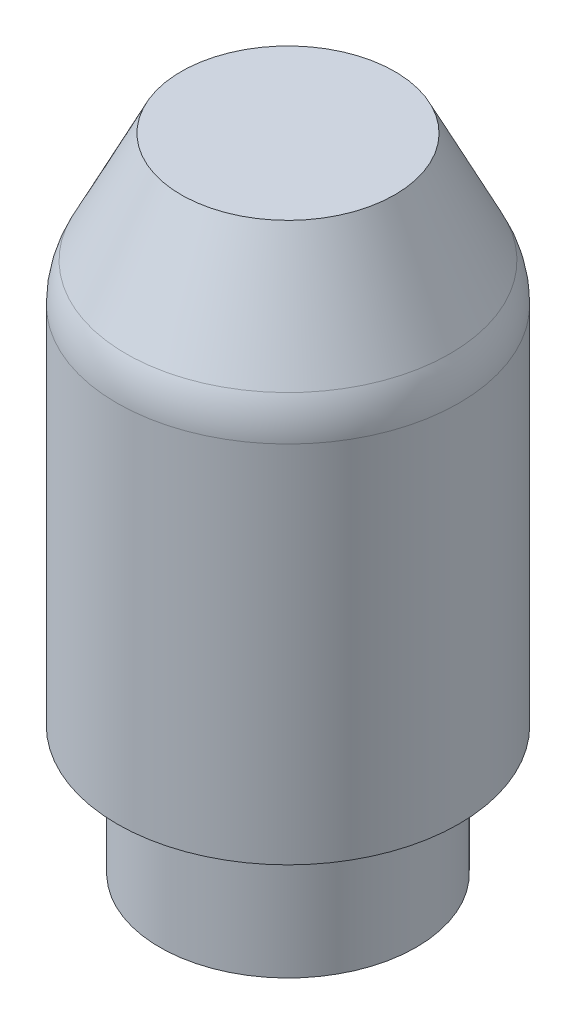
SolidWorks part; units mm, degrees
material "SKD11"
ref_plane "Front Plane" through (0, 0, 0) normal (0, 0, 1) x (1, 0, 0)
ref_plane "Top Plane" through (0, 0, 0) normal (0, 1, 0) x (1, 0, 0)
ref_plane "Right Plane" through (0, 0, 0) normal (1, 0, 0) x (0, 0, -1)
sketch "Sketch1" plane through (0, 0, 0) normal (0, 0, 1) x (1, 0, 0)
  line L0 (0, 0) -> (0, 15)
  line L1 (0, 15) -> (2.5, 15)
  line L2 (4, 12) -> (4, 3)
  line L3 (3, 0) -> (0, 0)
  line L4 (2.5, 15) -> (4, 12)
  line L5 (4, 3) -> (3, 3)
  line L6 (3, 3) -> (3, 0)
  dimension "D1" = 4
  dimension "D2" = 15
  dimension "D3" = 1.5
  dimension "D4" = 3
  dimension "D5" = 3
  dimension "D6" = 3
revolve "Revolve1" add sketch "Sketch1" angle 360 about L0
hole_wizard "M3 Tapped Hole1" positions "Sketch2" profile "Sketch3" tap size "M3" standard "ISO"
sketch "Sketch2" plane through (0, 0, 0) normal (0, -1, 0) x (-1, 0, 0)
  point P0 (0, 0)
sketch "Sketch3" plane through (0, 0, 0) normal (1, 0, 0) x (0, 0, -1)
  line L0 (0, 0) -> (0, 10.7511)
  line L1 (0, 10.7511) -> (1.25, 10)
  line L2 (1.25, 10) -> (1.25, 0)
  line L5 (1.25, 0) -> (0, 0)
  line L10 (0, 10.7511) -> (-1.25, 10) construction
  line L11 (0, -6.35) -> (0, 107.95) construction
  dimension "螺纹孔钻头直径" = 2.5
  dimension "螺纹孔钻头深度" = 10
  dimension "导头角度" = 118
cosmetic thread "Cosmetic thread 1" parameters "D1"=8, "D2"=3
fillet "Fillet1" radius 2 1 edges at (4, 12, 0)
